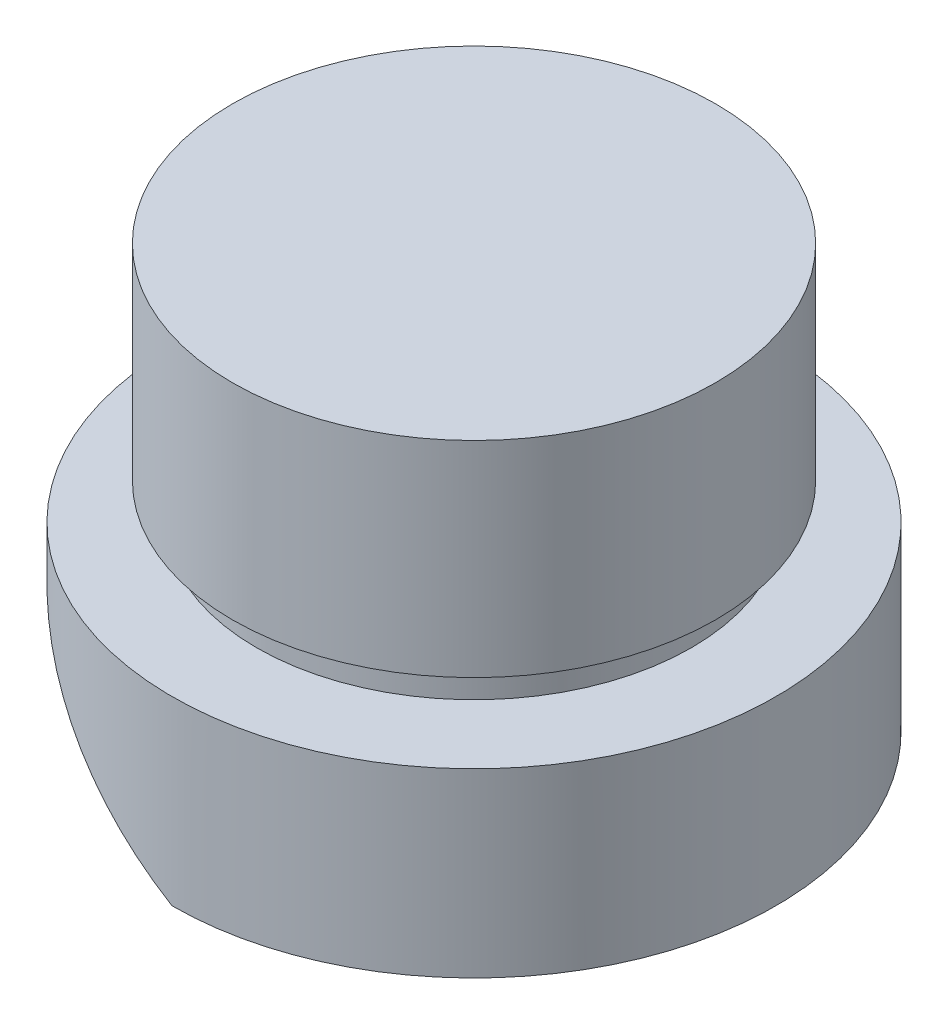
from build123d import *

# Parameters (mm, degrees)
SKETCH1_W               = 20
SKETCH1_H               = 17
SKETCH1_W_2             = 18
SKETCH1_H_2             = 3
CUT_EXTRUDE1_DEPTH      = 40.594796465
CUT_EXTRUDE1_DEPTH_BACK = 40.594796465


with BuildPart() as part:
    # Sketch1 → Revolve2 (revolve)
    with BuildSketch(Plane.XY, mode=Mode.PRIVATE) as revolve2_sk:
        with Locations((-10, 9.325484765)):
            Rectangle(SKETCH1_W, SKETCH1_H)
        with Locations((-9, -0.674515235)):
            Rectangle(SKETCH1_W_2, SKETCH1_H_2)
        Polygon((0, -17.174515235), (0, -2.174515235), (-18, -2.174515235), (-25, -2.174515235), (-25, -17.174515235), align=None)
    revolve(revolve2_sk.sketch.rotate(Axis((0, 13.711911357, 0), (0, -1, 0)), 270), axis=Axis((0, 13.711911357, 0), (0, -1, 0)))

    # Sketch3 → Cut-Extrude1 (cut, two sides: drawn at the far end of the back side and taken through both)
    with BuildSketch(Plane.XY.offset(-CUT_EXTRUDE1_DEPTH_BACK)):
        Polygon((-25, -2.174515235), (0, -17.174515235), (-25, -17.174515235), align=None)
    extrude(amount=CUT_EXTRUDE1_DEPTH + CUT_EXTRUDE1_DEPTH_BACK, mode=Mode.SUBTRACT)


solid = part.part
